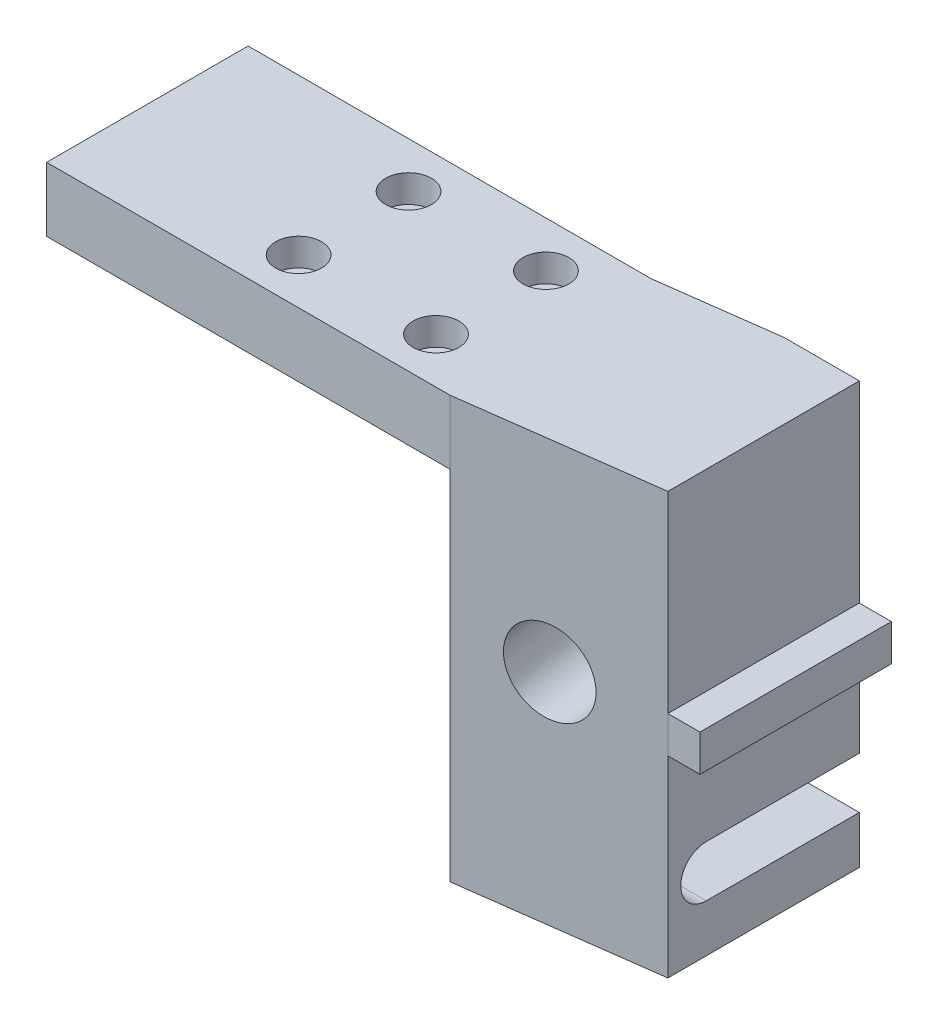
from build123d import *

# Parameters (mm, degrees)
SKETCH_1_W          = 68.51
SKETCH_1_H          = 46
EXTRUDE_1_DEPTH     = 23.69
CUT_EXTRUDE_1_REACH = 78.147
CUT_EXTRUDE_2_REACH = 72.493
CUT_EXTRUDE_3_REACH = 60.281
SKETCH_5_W          = 3.5
SKETCH_5_H          = 21
SKETCH_5_W_2        = 44.01
SKETCH_5_H_2        = 39
CUT_EXTRUDE_4_REACH = 59.946
SKETCH_6_R          = 4.5
CUT_EXTRUDE_5_REACH = 72.493
SKETCH_9_R          = 1.45
SKETCH_11_R         = 2.5
CUT_EXTRUDE_6_DEPTH = 3


with BuildPart() as part:
    # 草图1 → 凸台-拉伸1 (new body)
    with BuildSketch(Plane.XY):
        with Locations((-13.62, -0.3125)):
            Rectangle(SKETCH_1_W, SKETCH_1_H)
    extrude(amount=EXTRUDE_1_DEPTH)

    # 草图3 → 切除-拉伸1 (cut, up to next)
    with BuildSketch(Plane(origin=(20.635, 0, 0), x_dir=(0, 0, -1), z_dir=(1, 0, 0)), mode=Mode.PRIVATE) as cut_extrude_1_sk1:
        with BuildLine():
            Line((0, -18.1125), (-16.69, -18.1125))
            ThreePointArc((-16.69, -18.1125), (-19.49, -15.3125), (-16.69, -12.5125))
            Line((-16.69, -12.5125), (0, -12.5125))
            Line((0, -12.5125), (0, -18.1125))
        make_face()
    cut_extrude_1_tool1 = extrude(cut_extrude_1_sk1.sketch, amount=-CUT_EXTRUDE_1_REACH, mode=Mode.PRIVATE) & part.part
    add(cut_extrude_1_tool1.solids().sort_by_distance((20.635, -15.3125, 9.454896))[0], mode=Mode.SUBTRACT)

    # 草图4 → 切除-拉伸2 (cut, up to next)
    with BuildSketch(Plane(origin=(0, 22.6875, 0), x_dir=(1, 0, 0), z_dir=(0, 1, 0)), mode=Mode.PRIVATE) as cut_extrude_2_sk1:
        Polygon((20.635, -23.69), (20.635, -20.89), (17.135, -20.89), (-3.865, -23.69), align=None)
    cut_extrude_2_tool1 = extrude(cut_extrude_2_sk1.sketch, amount=-CUT_EXTRUDE_2_REACH, mode=Mode.PRIVATE) & part.part
    # 草图4 → 切除-拉伸2 (cut, up to next)
    with BuildSketch(Plane(origin=(0, 22.6875, 0), x_dir=(1, 0, 0), z_dir=(0, 1, 0)), mode=Mode.PRIVATE) as cut_extrude_2_sk2:
        Polygon((-47.875, 0), (-47.875, -1.7), (-3.875, -1.7), (8.925, 0), align=None)
    cut_extrude_2_tool2 = extrude(cut_extrude_2_sk2.sketch, amount=-CUT_EXTRUDE_2_REACH, mode=Mode.PRIVATE) & part.part
    add(cut_extrude_2_tool1.solids().sort_by_distance((12.3225, 22.6875, 22.64))[0], mode=Mode.SUBTRACT)
    add(cut_extrude_2_tool2.solids().sort_by_distance((-22.53955, 22.6875, 0.814021))[0], mode=Mode.SUBTRACT)

    # 草图5 → 切除-拉伸3 (cut, up to next)
    with BuildSketch(Plane.XY.offset(23.69), mode=Mode.PRIVATE) as cut_extrude_3_sk1:
        with Locations((18.885, -12.8125)):
            Rectangle(SKETCH_5_W, SKETCH_5_H)
    cut_extrude_3_tool1 = extrude(cut_extrude_3_sk1.sketch, amount=-CUT_EXTRUDE_3_REACH, mode=Mode.PRIVATE) & part.part
    # 草图5 → 切除-拉伸3 (cut, up to next)
    with BuildSketch(Plane.XY.offset(23.69), mode=Mode.PRIVATE) as cut_extrude_3_sk2:
        with Locations((18.885, 12.1875)):
            Rectangle(SKETCH_5_W, SKETCH_5_H)
    cut_extrude_3_tool2 = extrude(cut_extrude_3_sk2.sketch, amount=-CUT_EXTRUDE_3_REACH, mode=Mode.PRIVATE) & part.part
    # 草图5 → 切除-拉伸3 (cut, up to next)
    with BuildSketch(Plane.XY.offset(23.69), mode=Mode.PRIVATE) as cut_extrude_3_sk3:
        with Locations((-25.87, -3.8125)):
            Rectangle(SKETCH_5_W_2, SKETCH_5_H_2)
    cut_extrude_3_tool3 = extrude(cut_extrude_3_sk3.sketch, amount=-CUT_EXTRUDE_3_REACH, mode=Mode.PRIVATE) & part.part
    add(cut_extrude_3_tool1.solids().sort_by_distance((18.885, -12.8125, 23.69))[0], mode=Mode.SUBTRACT)
    add(cut_extrude_3_tool2.solids().sort_by_distance((18.885, 12.1875, 23.69))[0], mode=Mode.SUBTRACT)
    add(cut_extrude_3_tool3.solids().sort_by_distance((-25.87, -3.8125, 23.69))[0], mode=Mode.SUBTRACT)

    # 切除-拉伸4: up to this plane
    cut_extrude_4_end = Plane(origin=(17.135, -23.3135, 20.89), z_dir=(-0.13216372009101784, 0, -0.9912279006826348))
    # 草图6 → 切除-拉伸4 (cut, up to the surface)
    with BuildSketch(Plane(origin=(0.154700714, 0, 1.164805374), x_dir=(-0.9912954083909877, 0, 0.13165642142692813), z_dir=(-0.13165642142692813, 0, -0.9912954083909877)), mode=Mode.PRIVATE) as cut_extrude_4_sk1:
        with Locations((-2.755002186, 0.6875)):
            Circle(SKETCH_6_R)
    cut_extrude_4_tool1 = split(extrude(cut_extrude_4_sk1.sketch, amount=-CUT_EXTRUDE_4_REACH, mode=Mode.PRIVATE), bisect_by=cut_extrude_4_end, keep=Keep.BOTH, mode=Mode.PRIVATE)
    add(cut_extrude_4_tool1.solids().sort_by_distance((2.885722, 0.6875, 0.802092))[0], mode=Mode.SUBTRACT)

    # 草图9 → 切除-拉伸5 (cut, up to next)
    with BuildSketch(Plane(origin=(0, 22.6875, 0), x_dir=(1, 0, 0), z_dir=(0, 1, 0)), mode=Mode.PRIVATE) as cut_extrude_5_sk1:
        with Locations(Location((-25.375, -6.69, 0), (0, 0, 270))):
            Circle(SKETCH_9_R)
    cut_extrude_5_tool1 = extrude(cut_extrude_5_sk1.sketch, amount=-CUT_EXTRUDE_5_REACH, mode=Mode.PRIVATE) & part.part
    # 草图9 → 切除-拉伸5 (cut, up to next)
    with BuildSketch(Plane(origin=(0, 22.6875, 0), x_dir=(1, 0, 0), z_dir=(0, 1, 0)), mode=Mode.PRIVATE) as cut_extrude_5_sk2:
        with Locations(Location((-25.375, -18.69, 0), (0, 0, 270))):
            Circle(SKETCH_9_R)
    cut_extrude_5_tool2 = extrude(cut_extrude_5_sk2.sketch, amount=-CUT_EXTRUDE_5_REACH, mode=Mode.PRIVATE) & part.part
    # 草图9 → 切除-拉伸5 (cut, up to next)
    with BuildSketch(Plane(origin=(0, 22.6875, 0), x_dir=(1, 0, 0), z_dir=(0, 1, 0)), mode=Mode.PRIVATE) as cut_extrude_5_sk3:
        with Locations(Location((-10.375, -18.69, 0), (0, 0, 270))):
            Circle(SKETCH_9_R)
    cut_extrude_5_tool3 = extrude(cut_extrude_5_sk3.sketch, amount=-CUT_EXTRUDE_5_REACH, mode=Mode.PRIVATE) & part.part
    # 草图9 → 切除-拉伸5 (cut, up to next)
    with BuildSketch(Plane(origin=(0, 22.6875, 0), x_dir=(1, 0, 0), z_dir=(0, 1, 0)), mode=Mode.PRIVATE) as cut_extrude_5_sk4:
        with Locations(Location((-10.375, -6.69, 0), (0, 0, 270))):
            Circle(SKETCH_9_R)
    cut_extrude_5_tool4 = extrude(cut_extrude_5_sk4.sketch, amount=-CUT_EXTRUDE_5_REACH, mode=Mode.PRIVATE) & part.part
    add(cut_extrude_5_tool1.solids().sort_by_distance((-25.375, 22.6875, 6.69))[0], mode=Mode.SUBTRACT)
    add(cut_extrude_5_tool2.solids().sort_by_distance((-25.375, 22.6875, 18.69))[0], mode=Mode.SUBTRACT)
    add(cut_extrude_5_tool3.solids().sort_by_distance((-10.375, 22.6875, 18.69))[0], mode=Mode.SUBTRACT)
    add(cut_extrude_5_tool4.solids().sort_by_distance((-10.375, 22.6875, 6.69))[0], mode=Mode.SUBTRACT)

    # 草图11 → 切除-拉伸6 (cut)
    with BuildSketch(Plane(origin=(0, 22.6875, 0), x_dir=(1, 0, 0), z_dir=(0, 1, 0))):
        with Locations(Location((-25.375, -6.69, 0), (0, 0, 270))):
            Circle(SKETCH_11_R)
        with Locations(Location((-10.375, -6.69, 0), (0, 0, 270))):
            Circle(SKETCH_11_R)
        with Locations(Location((-25.375, -18.69, 0), (0, 0, 270))):
            Circle(SKETCH_11_R)
        with Locations(Location((-10.375, -18.69, 0), (0, 0, 270))):
            Circle(SKETCH_11_R)
    extrude(amount=-CUT_EXTRUDE_6_DEPTH, mode=Mode.SUBTRACT)


solid = part.part
